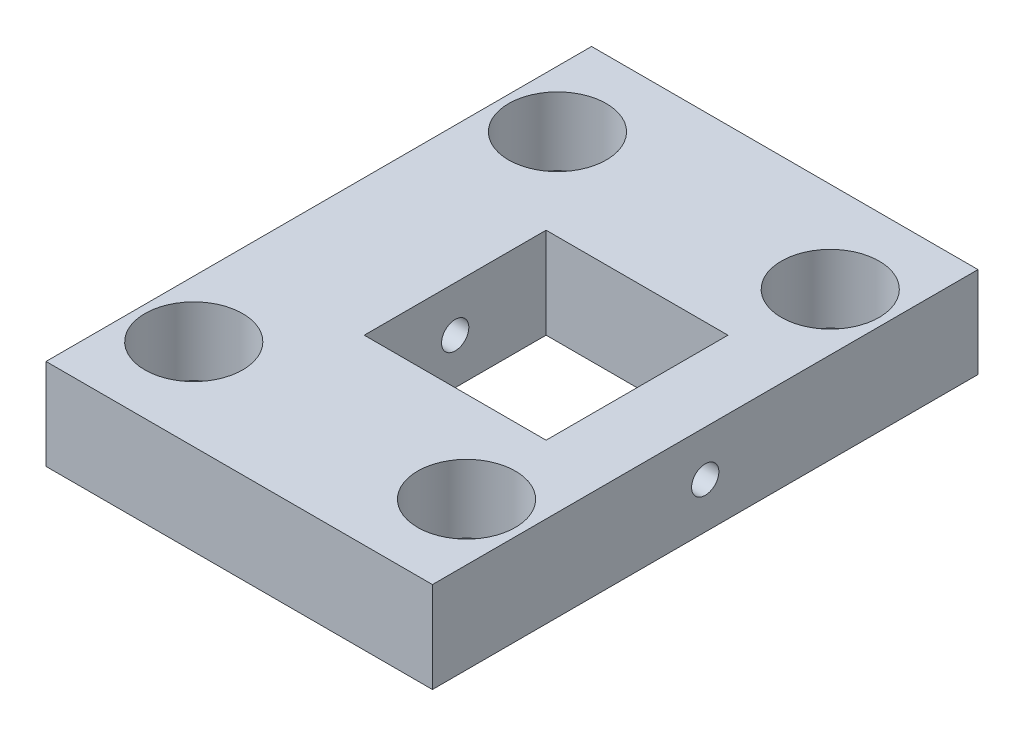
SolidWorks part; units mm, degrees
ref_plane "Front Plane" through (0, 0, 0) normal (0, 0, 1) x (1, 0, 0)
ref_plane "Top Plane" through (0, 0, 0) normal (0, 1, 0) x (1, 0, 0)
ref_plane "Right Plane" through (0, 0, 0) normal (1, 0, 0) x (0, 0, -1)
sketch "Sketch1" plane through (0, 0, 0) normal (0, 1, 0) x (1, 0, 0)
  line L1 (-42.5, -60) -> (42.5, -60)
  line L2 (-42.5, -60) -> (-42.5, 60)
  line L3 (-42.5, 60) -> (42.5, 60)
  line L4 (42.5, -60) -> (42.5, 60)
  line L5 (-42.5, -60) -> (42.5, 60) construction
  line L6 (-42.5, 60) -> (42.5, -60) construction
  line L7 (-30, -40) -> (30, -40) construction
  line L8 (-30, -40) -> (-30, 40) construction
  line L9 (-30, 40) -> (30, 40) construction
  line L10 (30, -40) -> (30, 40) construction
  line L11 (-30, -40) -> (30, 40) construction
  line L12 (-30, 40) -> (30, -40) construction
  line L13 (-12.5, -20) -> (27.5, -20)
  line L14 (-12.5, -20) -> (-12.5, 20)
  line L15 (-12.5, 20) -> (27.5, 20)
  line L16 (27.5, -20) -> (27.5, 20)
  line L17 (-12.5, -20) -> (27.5, 20) construction
  line L18 (-12.5, 20) -> (27.5, -20) construction
  circle A0 centre (-30, 40) radius 5.5
  circle A1 centre (30, 40) radius 5.5
  circle A2 centre (30, -40) radius 5.5
  circle A3 centre (-30, -40) radius 5.5
  point P0 (0, 0)
  point P5 (0, 0)
  point P15 (7.5, 0)
  dimension "D5" = 11
  dimension "D6" = 11
  dimension "D7" = 11
  dimension "D8" = 11
  dimension "D1" = 85
  dimension "D2" = 120
  dimension "D3" = 80
  dimension "D4" = 60
  dimension "D9" = 40
  dimension "D10" = 40
  dimension "D11" = 35
extrude "Boss-Extrude1" add sketch "Sketch1" along normal blind 20
sketch "Sketch2" plane through (0, 20, 0) normal (0, 1, 0) x (1, 0, 0)
  circle A0 centre (30, 40) radius 10.75
  circle A1 centre (-30, 40) radius 10.75
  circle A2 centre (-30, -40) radius 10.75
  circle A3 centre (30, -40) radius 10.75
  dimension "D1" = 21.5
  dimension "D2" = 21.5
  dimension "D3" = 21.5
  dimension "D4" = 21.5
extrude "Cut-Extrude1" cut sketch "Sketch2" against normal blind 15
sketch "Sketch3" plane through (-42.5, 0, 0) normal (-1, 0, 0) x (0, 0, 1)
  line L0 (-60, 20) -> (60, 20) construction
  circle A0 centre (0, 10) radius 3
  dimension "D1" = 6
  dimension "D2" = 10
extrude "Cut-Extrude2" cut sketch "Sketch3" against normal through all
